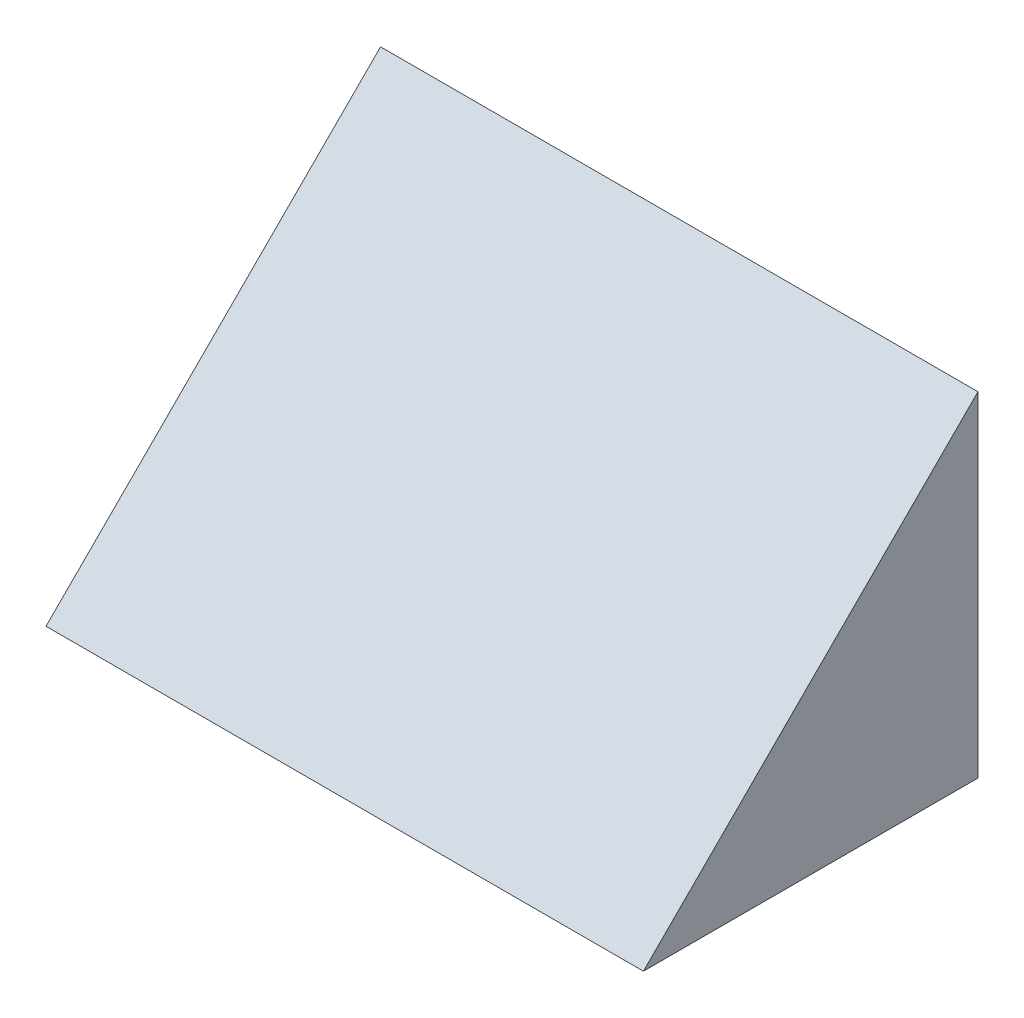
SolidWorks part; units mm, degrees
ref_plane "Front" through (0, 0, 0) normal (0, 0, 1) x (1, 0, 0)
ref_plane "Top" through (0, 0, 0) normal (0, 1, 0) x (1, 0, 0)
ref_plane "Right" through (0, 0, 0) normal (1, 0, 0) x (0, 0, -1)
sketch "Sketch1" plane through (0, 0, 0) normal (0, 0, 1) x (1, 0, 0)
  line L1 (40, 200) -> (-40, 200)
  line L2 (40, 200) -> (40, -200)
  line L3 (40, -200) -> (-40, -200)
  line L4 (-40, 200) -> (-40, -200)
  line L5 (40, 200) -> (-40, -200) construction
  line L6 (40, -200) -> (-40, 200) construction
  point P0 (0, 0)
  dimension "D1" = 400
  dimension "D2" = 80
extrude "Boss-Extrude1" add sketch "Sketch1" along normal blind 80
sketch "Sketch2" plane through (-40, 0, 0) normal (-1, 0, 0) x (0, 0, 1)
  line L0 (0, -200) -> (400, -200)
  line L2 (400, -200) -> (0, 200)
  line L3 (0, 200) -> (0, -200)
  dimension "D1" = 400
extrude "Boss-Extrude2" add sketch "Sketch2" against normal up to surface (80 mm away) up to face at (40, 0, 40)
sketch "Sketch3" plane through (-40, 0, 0) normal (-1, 0, 0) x (0, 0, 1)
  line L0 (80, 120) -> (0, 200)
  line L1 (0, 200) -> (0, -200) construction
  line L2 (0, 200) -> (172.988, 200)
  line L3 (172.988, 200) -> (80, 120)
extrude "Cut-Extrude1" cut sketch "Sketch3" against normal blind 300
sketch "Sketch4" plane through (-40, 0, 0) normal (-1, 0, 0) x (0, 0, 1)
  line L0 (0, -200) -> (0, 250)
  line L1 (0, -200) -> (450, -200)
  line L2 (450, -200) -> (0, 250)
  dimension "D1" = 450
  dimension "D2" = 450
extrude "Boss-Extrude3" add sketch "Sketch4" against normal blind 500
sketch "Sketch5" plane through (-40, 0, 0) normal (-1, 0, 0) x (0, 0, 1)
  line L1 (450, -200) -> (0, -200) construction
  line L2 (280, -200) -> (0, 80)
  line L3 (0, 250) -> (0, -200) construction
  line L5 (280, -200) -> (450, -200)
  line L6 (450, -200) -> (0, 250)
  line L7 (0, 250) -> (0, 80)
  dimension "D1" = 170
  dimension "D2" = 170
extrude "Cut-Extrude2" cut sketch "Sketch5" against normal through all both and the other way through all
